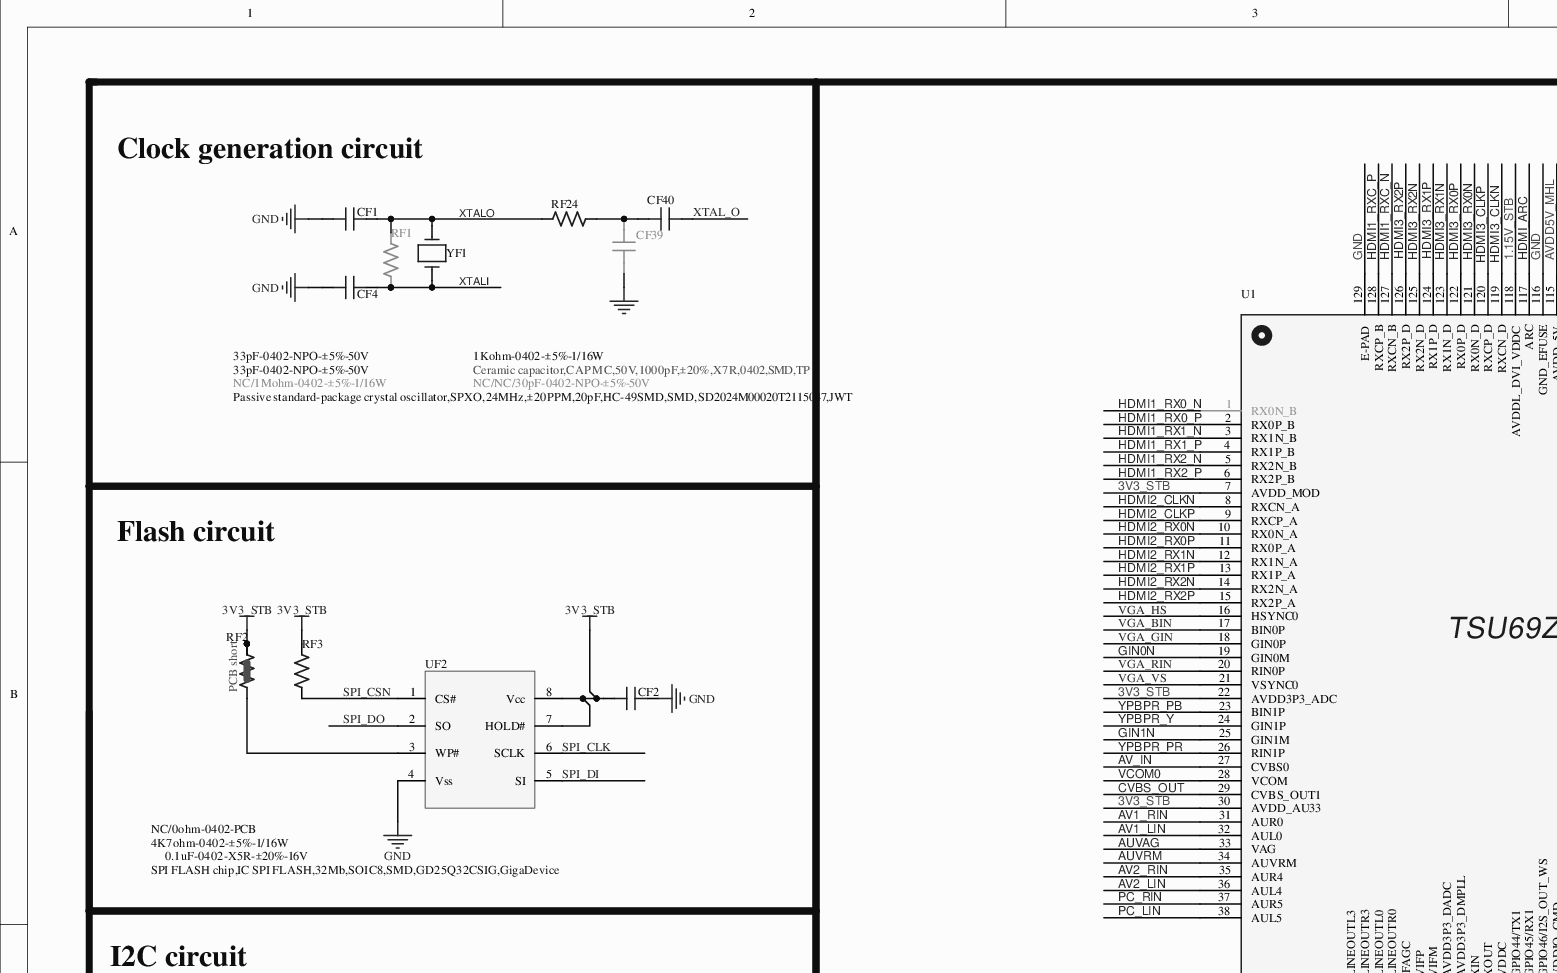
[diagram p0: MISC84438-8.SchDoc, top left]
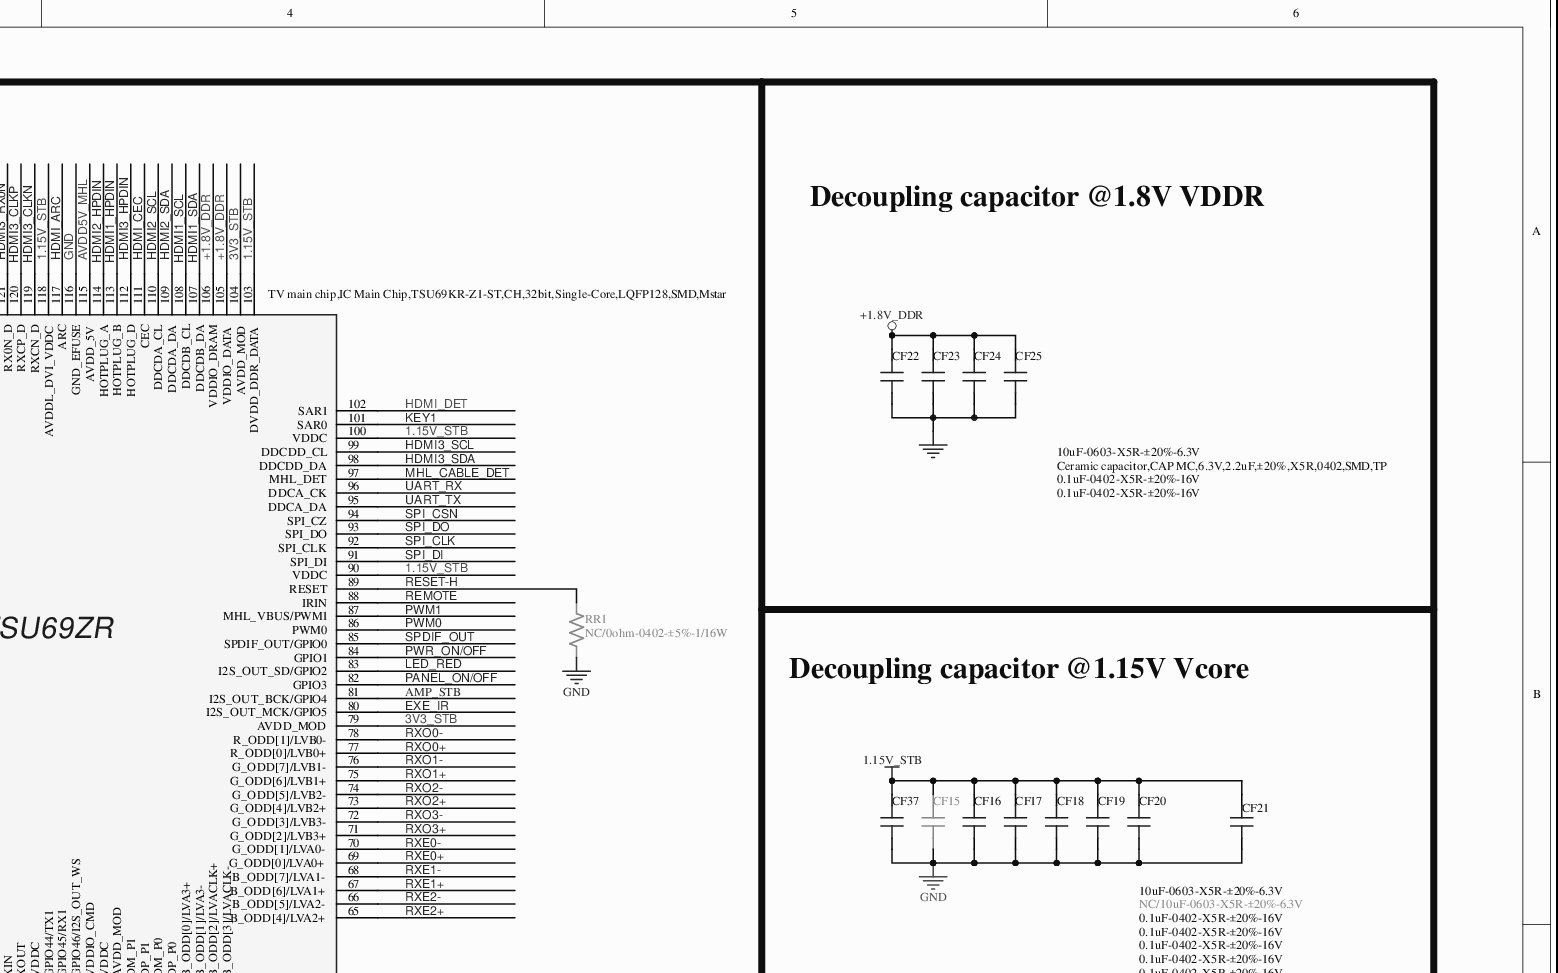
[diagram p1: MISC84438-8.SchDoc, top right]
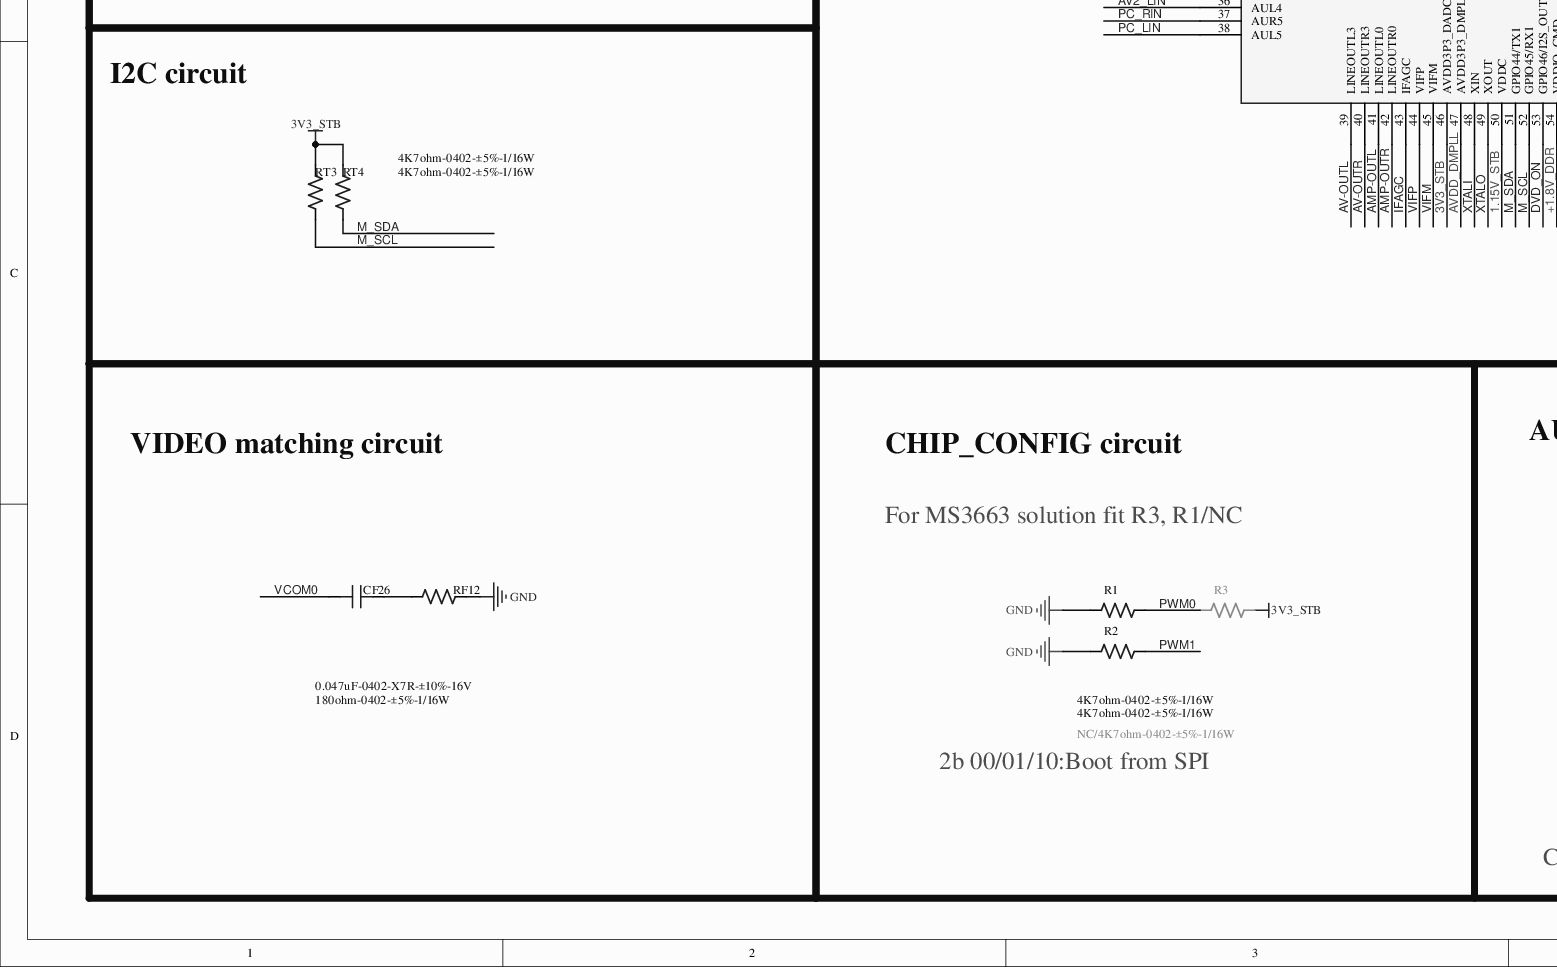
[diagram p2: MISC84438-8.SchDoc, bottom left]
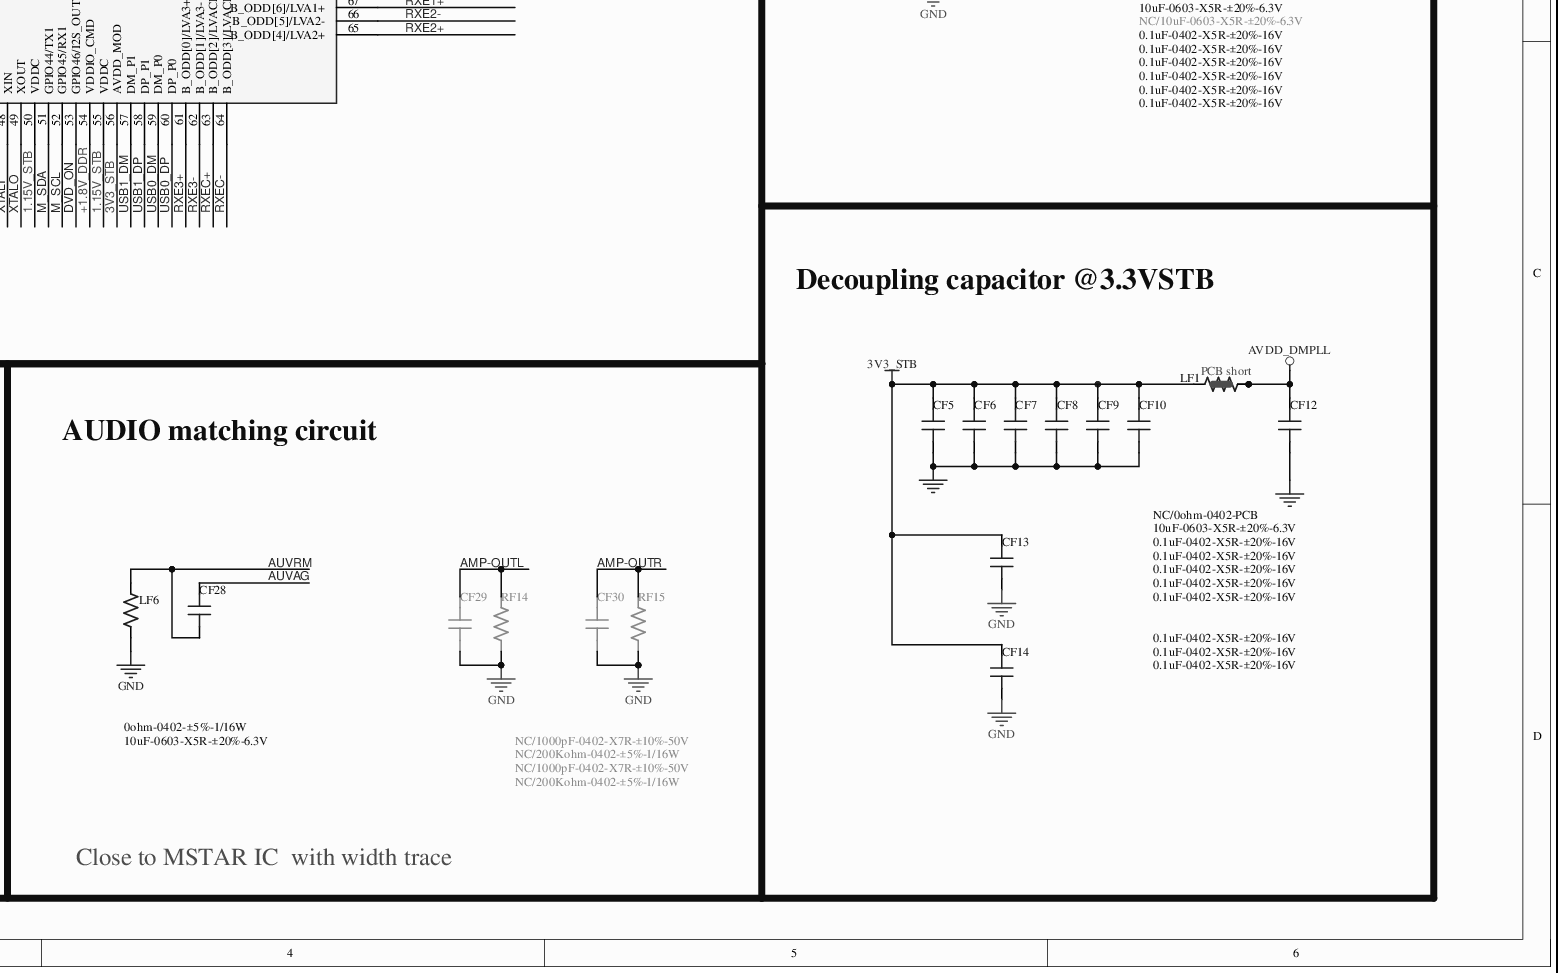
[diagram p3: MISC84438-8.SchDoc, bottom right]
# Altium project MISC84438-18.PrjPCB (part 4 of 8)

## Sheet MISC84438-8.SchDoc
size 558 x 342 mm

### Parts
CF1  33pF-0402-NPO-±5%-50V  [C0402]
CF2  0.1uF-0402-X5R-±20%-16V  [C0402]
CF4  33pF-0402-NPO-±5%-50V  [C0402]
CF5  10uF-0603-X5R-±20%-6.3V  [C0603]
CF6  0.1uF-0402-X5R-±20%-16V  [C0402]
CF7  0.1uF-0402-X5R-±20%-16V  [C0402]
CF8  0.1uF-0402-X5R-±20%-16V  [C0402]
CF9  0.1uF-0402-X5R-±20%-16V  [C0402]
CF10  0.1uF-0402-X5R-±20%-16V  [C0402]
CF12  0.1uF-0402-X5R-±20%-16V  [C0402]
CF13  0.1uF-0402-X5R-±20%-16V  [C0402]
CF14  0.1uF-0402-X5R-±20%-16V  [C0402]
CF15  NC/10uF-0603-X5R-±20%-6.3V  [C0603]
CF16  0.1uF-0402-X5R-±20%-16V  [C0402]
CF17  0.1uF-0402-X5R-±20%-16V  [C0402]
CF18  0.1uF-0402-X5R-±20%-16V  [C0402]
CF19  0.1uF-0402-X5R-±20%-16V  [C0402]
CF20  0.1uF-0402-X5R-±20%-16V  [C0402]
CF21  0.1uF-0402-X5R-±20%-16V  [C0402]
CF22  10uF-0603-X5R-±20%-6.3V  [C0603]
CF23  Ceramic capacitor,CAP MC,6.3V,2.2uF,±20%,X5R,0402,SMD,TP  [C0402]
CF24  0.1uF-0402-X5R-±20%-16V  [C0402]
CF25  0.1uF-0402-X5R-±20%-16V  [C0402]
CF26  0.047uF-0402-X7R-±10%-16V  [C0402]
CF28  10uF-0603-X5R-±20%-6.3V  [C0603]
CF29  NC/1000pF-0402-X7R-±10%-50V  [C0402]
CF30  NC/1000pF-0402-X7R-±10%-50V  [C0402]
CF37  10uF-0603-X5R-±20%-6.3V  [C0603]
CF39  NC/NC/30pF-0402-NPO-±5%-50V  [C0402]
CF40  Ceramic capacitor,CAP MC,50V,1000pF,±20%,X7R,0402,SMD,TP  [C0402]
LF1  NC/0ohm-0402-PCB  [R0402SC]
LF6  0ohm-0402-±5%-1/16W  [R0402]
R1  4K7ohm-0402-±5%-1/16W  [R0402]
R2  4K7ohm-0402-±5%-1/16W  [R0402]
R3  NC/4K7ohm-0402-±5%-1/16W  [R0402]
RF1  NC/1Mohm-0402-±5%-1/16W  [R0402]
RF2  NC/0ohm-0402-PCB  [R0402SC]
RF3  4K7ohm-0402-±5%-1/16W  [R0402]
RF12  180ohm-0402-±5%-1/16W  [R0402]
RF14  NC/200Kohm-0402-±5%-1/16W  [R0402]
RF15  NC/200Kohm-0402-±5%-1/16W  [R0402]
RF24  1Kohm-0402-±5%-1/16W  [R0402]
RR1  NC/0ohm-0402-±5%-1/16W  [R0402]
RT3  4K7ohm-0402-±5%-1/16W  [R0402]
RT4  4K7ohm-0402-±5%-1/16W  [R0402]
U1  TV main chip,IC Main Chip,TSU69KR-Z1-ST,CH,32bit,Single-Core,LQFP128,SMD,Mstar  [QFP128/0.4-5]
UF2  SPI FLASH chip,IC SPI FLASH,32Mb,SOIC8,SMD,GD25Q32CSIG,GigaDevice  [SOIC8]
YF1  Passive standard-package crystal oscillator,SPXO,24MHz,±20PPM,20pF,HC-49SMD,SMD,SD2024M00020T2115047,JWT  [XTAL-S-1]

### Blocks framed on the sheet
Flash circuit: CF2 RF2 RF3 UF2
VIDEO matching circuit: CF26 RF12

### Nets
1.15V_STB: CF15.1 CF16.2 CF17.2 CF18.2 CF19.2 CF20.2 CF21.2 CF37.1 U1.50(VDDC) U1.55(VDDC) U1.90(VDDC) U1.100(VDDC) U1.103(DVDD_DDR_DATA) U1.118(AVDDL_DVI_VDDC)
3V3_STB: CF2.2 CF5.1 CF6.2 CF7.2 CF8.2 CF9.2 CF10.2 CF13.2 CF14.2 LF1.1 R3.2 RF2.2 RF2.3 RF3.2 RT3.1 RT4.1 U1.7(AVDD_MOD) U1.22(AVDD3P3_ADC) U1.30(AVDD_AU33) U1.46(AVDD3P3_DADC) U1.56(AVDD_MOD) U1.79(AVDD_MOD) U1.104(AVDD_MOD) UF2.7(HOLD#) UF2.8(Vcc)
+1.8V_DDR: CF22.1 CF23.2 CF24.2 CF25.2 U1.54(VDDIO_CMD) U1.105(VDDIO_DATA) U1.106(VDDIO_DRAM)
AVDD_DMPLL: CF12.2 LF1.2 LF1.3 U1.47(AVDD3P3_DMPLL)
GND: CF1.1 CF2.1 CF4.1 CF5.2 CF6.1 CF7.1 CF8.1 CF9.1 CF10.1 CF12.1 CF13.1 CF14.1 CF15.2 CF16.1 CF17.1 CF18.1 CF19.1 CF20.1 CF21.1 CF22.2 CF23.1 CF24.1 CF25.1 CF29.2 CF30.2 CF37.2 CF39.1 LF6.1 R1.2 R2.2 RF12.2 RF14.1 RF15.1 RR1.1 U1.116(GND_EFUSE) U1.129(E-PAD) UF2.4(Vss)
AMP-OUTL: CF29.1 RF14.2 U1.41(LINEOUTL0)
AMP-OUTR: CF30.1 RF15.2 U1.42(LINEOUTR0)
AMP_STB: U1.81(I2S_OUT_BCK/GPIO4)
AUVAG: CF28.2 U1.33(VAG)
AUVRM: CF28.1 LF6.2 U1.34(AUVRM)
AV1_LIN: U1.32(AUL0)
AV1_RIN: U1.31(AUR0)
AV2_LIN: U1.36(AUL4)
AV2_RIN: U1.35(AUR4)
AV-OUTL: U1.39(LINEOUTL3)
AV-OUTR: U1.40(LINEOUTR3)
AV_IN: U1.27(CVBS0)
AVDD5V_MHL: U1.115(AVDD_5V)
CVBS_OUT: U1.29(CVBS_OUT1)
DVD_ON: U1.53(GPIO46/I2S_OUT_WS)
EXE_IR: U1.80(I2S_OUT_MCK/GPIO5)
GIN0N: U1.19(GIN0M)
GIN1N: U1.25(GIN1M)
HDMI1_HPDIN: U1.113(HOTPLUG_B)
HDMI1_RX0_N: U1.1(RX0N_B)
HDMI1_RX0_P: U1.2(RX0P_B)
HDMI1_RX1_N: U1.3(RX1N_B)
HDMI1_RX1_P: U1.4(RX1P_B)
HDMI1_RX2_N: U1.5(RX2N_B)
HDMI1_RX2_P: U1.6(RX2P_B)
HDMI1_RXC_N: U1.127(RXCN_B)
HDMI1_RXC_P: U1.128(RXCP_B)
HDMI1_SCL: U1.108(DDCDB_CL)
HDMI1_SDA: U1.107(DDCDB_DA)
HDMI2_CLKN: U1.8(RXCN_A)
HDMI2_CLKP: U1.9(RXCP_A)
HDMI2_HPDIN: U1.114(HOTPLUG_A)
HDMI2_RX0N: U1.10(RX0N_A)
HDMI2_RX0P: U1.11(RX0P_A)
HDMI2_RX1N: U1.12(RX1N_A)
HDMI2_RX1P: U1.13(RX1P_A)
HDMI2_RX2N: U1.14(RX2N_A)
HDMI2_RX2P: U1.15(RX2P_A)
HDMI2_SCL: U1.110(DDCDA_CL)
HDMI2_SDA: U1.109(DDCDA_DA)
HDMI3_CLKN: U1.119(RXCN_D)
HDMI3_CLKP: U1.120(RXCP_D)
HDMI3_HPDIN: U1.112(HOTPLUG_D)
HDMI3_RX0N: U1.121(RX0N_D)
HDMI3_RX0P: U1.122(RX0P_D)
HDMI3_RX1N: U1.123(RX1N_D)
HDMI3_RX1P: U1.124(RX1P_D)
HDMI3_RX2N: U1.125(RX2N_D)
HDMI3_RX2P: U1.126(RX2P_D)
HDMI3_SCL: U1.99(DDCDD_CL)
HDMI3_SDA: U1.98(DDCDD_DA)
HDMI_ARC: U1.117(ARC)
HDMI_CEC: U1.111(CEC)
HDMI_DET: U1.102(SAR1)
IFAGC: U1.43(IFAGC)
KEY1: U1.101(SAR0)
LED_RED: U1.83(I2S_OUT_SD/GPIO2)
M_SCL: RT3.2 U1.52(GPIO45/RX1)
M_SDA: RT4.2 U1.51(GPIO44/TX1)
MHL_CABLE_DET: U1.97(MHL_DET)
PANEL_ON/OFF: U1.82(GPIO3)
PC_LIN: U1.38(AUL5)
PC_RIN: U1.37(AUR5)
PWM0: R1.1 R3.1 U1.86(PWM0)
PWM1: R2.1 U1.87(MHL_VBUS/PWM1)
PWR_ON/OFF: U1.84(GPIO1)
REMOTE: U1.88(IRIN)
RESET-H: RR1.2 U1.89(RESET)
RXE0+: U1.69(G_ODD[0]/LVA0+)
RXE0-: U1.70(G_ODD[1]/LVA0-)
RXE1+: U1.67(B_ODD[6]/LVA1+)
RXE1-: U1.68(B_ODD[7]/LVA1-)
RXE2+: U1.65(B_ODD[4]/LVA2+)
RXE2-: U1.66(B_ODD[5]/LVA2-)
RXE3+: U1.61(B_ODD[0]/LVA3+)
RXE3-: U1.62(B_ODD[1]/LVA3-)
RXEC+: U1.63(B_ODD[2]/LVACLK+)
RXEC-: U1.64(B_ODD[3]/LVACLK-)
RXO0+: U1.77(R_ODD[0]/LVB0+)
RXO0-: U1.78(R_ODD[1]/LVB0-)
RXO1+: U1.75(G_ODD[6]/LVB1+)
RXO1-: U1.76(G_ODD[7]/LVB1-)
RXO2+: U1.73(G_ODD[4]/LVB2+)
RXO2-: U1.74(G_ODD[5]/LVB2-)
RXO3+: U1.71(G_ODD[2]/LVB3+)
RXO3-: U1.72(G_ODD[3]/LVB3-)
SPDIF_OUT: U1.85(SPDIF_OUT/GPIO0)
SPI_CLK: U1.92(SPI_CLK) UF2.6(SCLK)
SPI_CSN: RF3.1 U1.94(SPI_CZ) UF2.1(CS#)
SPI_DI: U1.91(SPI_DI) UF2.5(SI)
SPI_DO: U1.93(SPI_DO) UF2.2(SO)
UART_RX: U1.96(DDCA_CK)
UART_TX: U1.95(DDCA_DA)
USB0_DM: U1.59(DM_P0)
USB0_DP: U1.60(DP_P0)
USB1_DM: U1.57(DM_P1)
USB1_DP: U1.58(DP_P1)
VCOM0: CF26.1 U1.28(VCOM)
VGA_BIN: U1.17(BIN0P)
VGA_GIN: U1.18(GIN0P)
VGA_HS: U1.16(HSYNC0)
VGA_RIN: U1.20(RIN0P)
VGA_VS: U1.21(VSYNC0)
VIFM: U1.45(VIFM)
VIFP: U1.44(VIFP)
XTAL_O: CF40.1
XTALI: CF4.2 RF1.1 U1.48(XIN) YF1.1
XTALO: CF1.2 RF1.2 RF24.2 U1.49(XOUT) YF1.2
YPBPR_PB: U1.23(BIN1P)
YPBPR_PR: U1.26(RIN1P)
YPBPR_Y: U1.24(GIN1P)
NetCF26_2: CF26.2 RF12.1
NetCF39_2: CF39.2 CF40.2 RF24.1
NetRF2_1: RF2.1 UF2.3(WP#)

### Notes on the sheet
- Clock generation circuit
- Decoupling capacitor @1.8V VDDR
- Decoupling capacitor @1.15V Vcore
- I2C circuit
- Decoupling capacitor @3.3VSTB
- AUDIO matching circuit
- CHIP_CONFIG circuit
- For MS3663 solution fit R3, R1/NC
- 2b 00/01/10:Boot from SPI
- Close to MSTAR IC  with width trace

### Library data of the parts
CF1 CF4 = 33pF-0402-NPO-±5%-50V-D
CF2 CF7-CF10 CF12-CF14 CF17 = 0.1uF-0402-Y5V-+80%-20%-16V-D
CF5 CF15 CF22 CF28 CF37 = 10uF-0603-X5R-±20%-6.3V-D
CF6 CF16 CF18-CF21 CF23-CF25 = 1uF-0402-X5R-±20%-6.3V-D
CF26 = 0.047uF-0402-X7R-±10%-16V-D
CF29 CF30 = 1000pF-0402-X7R-±10%-50V-D
CF39 CF40 = 30pF-0402-NPO-±5%-50V-D
LF1 RF2 = 0ohm-0402-PCB-D
LF6 RR1 = 0ohm-0402-±5%-1/16W-D
R1-R3 RF3 RT3 RT4 = 4K7ohm-0402-±5%-1/16W-D
RF1 = 1Mohm-0402-±5%-1/16W-D
RF12 = 68ohm-0402-±5%-1/16W-D
RF14 RF15 = 200Kohm-0402-±5%-1/16W-D
RF24 = 1Kohm-0402-±5%-1/16W-D
U1 = TSU69ZR-D
UF2 = SPI FLASH 芯片,IC SPI FLASH,32Mb,SOIC8,SMD,GD25Q32CSIG,GigaDevice-D
YF1 = 24MHz-±20PPM-20PF-HC-49S-SMD-D

## Sheet MISC84438-9.SchDoc
size 431 x 292 mm
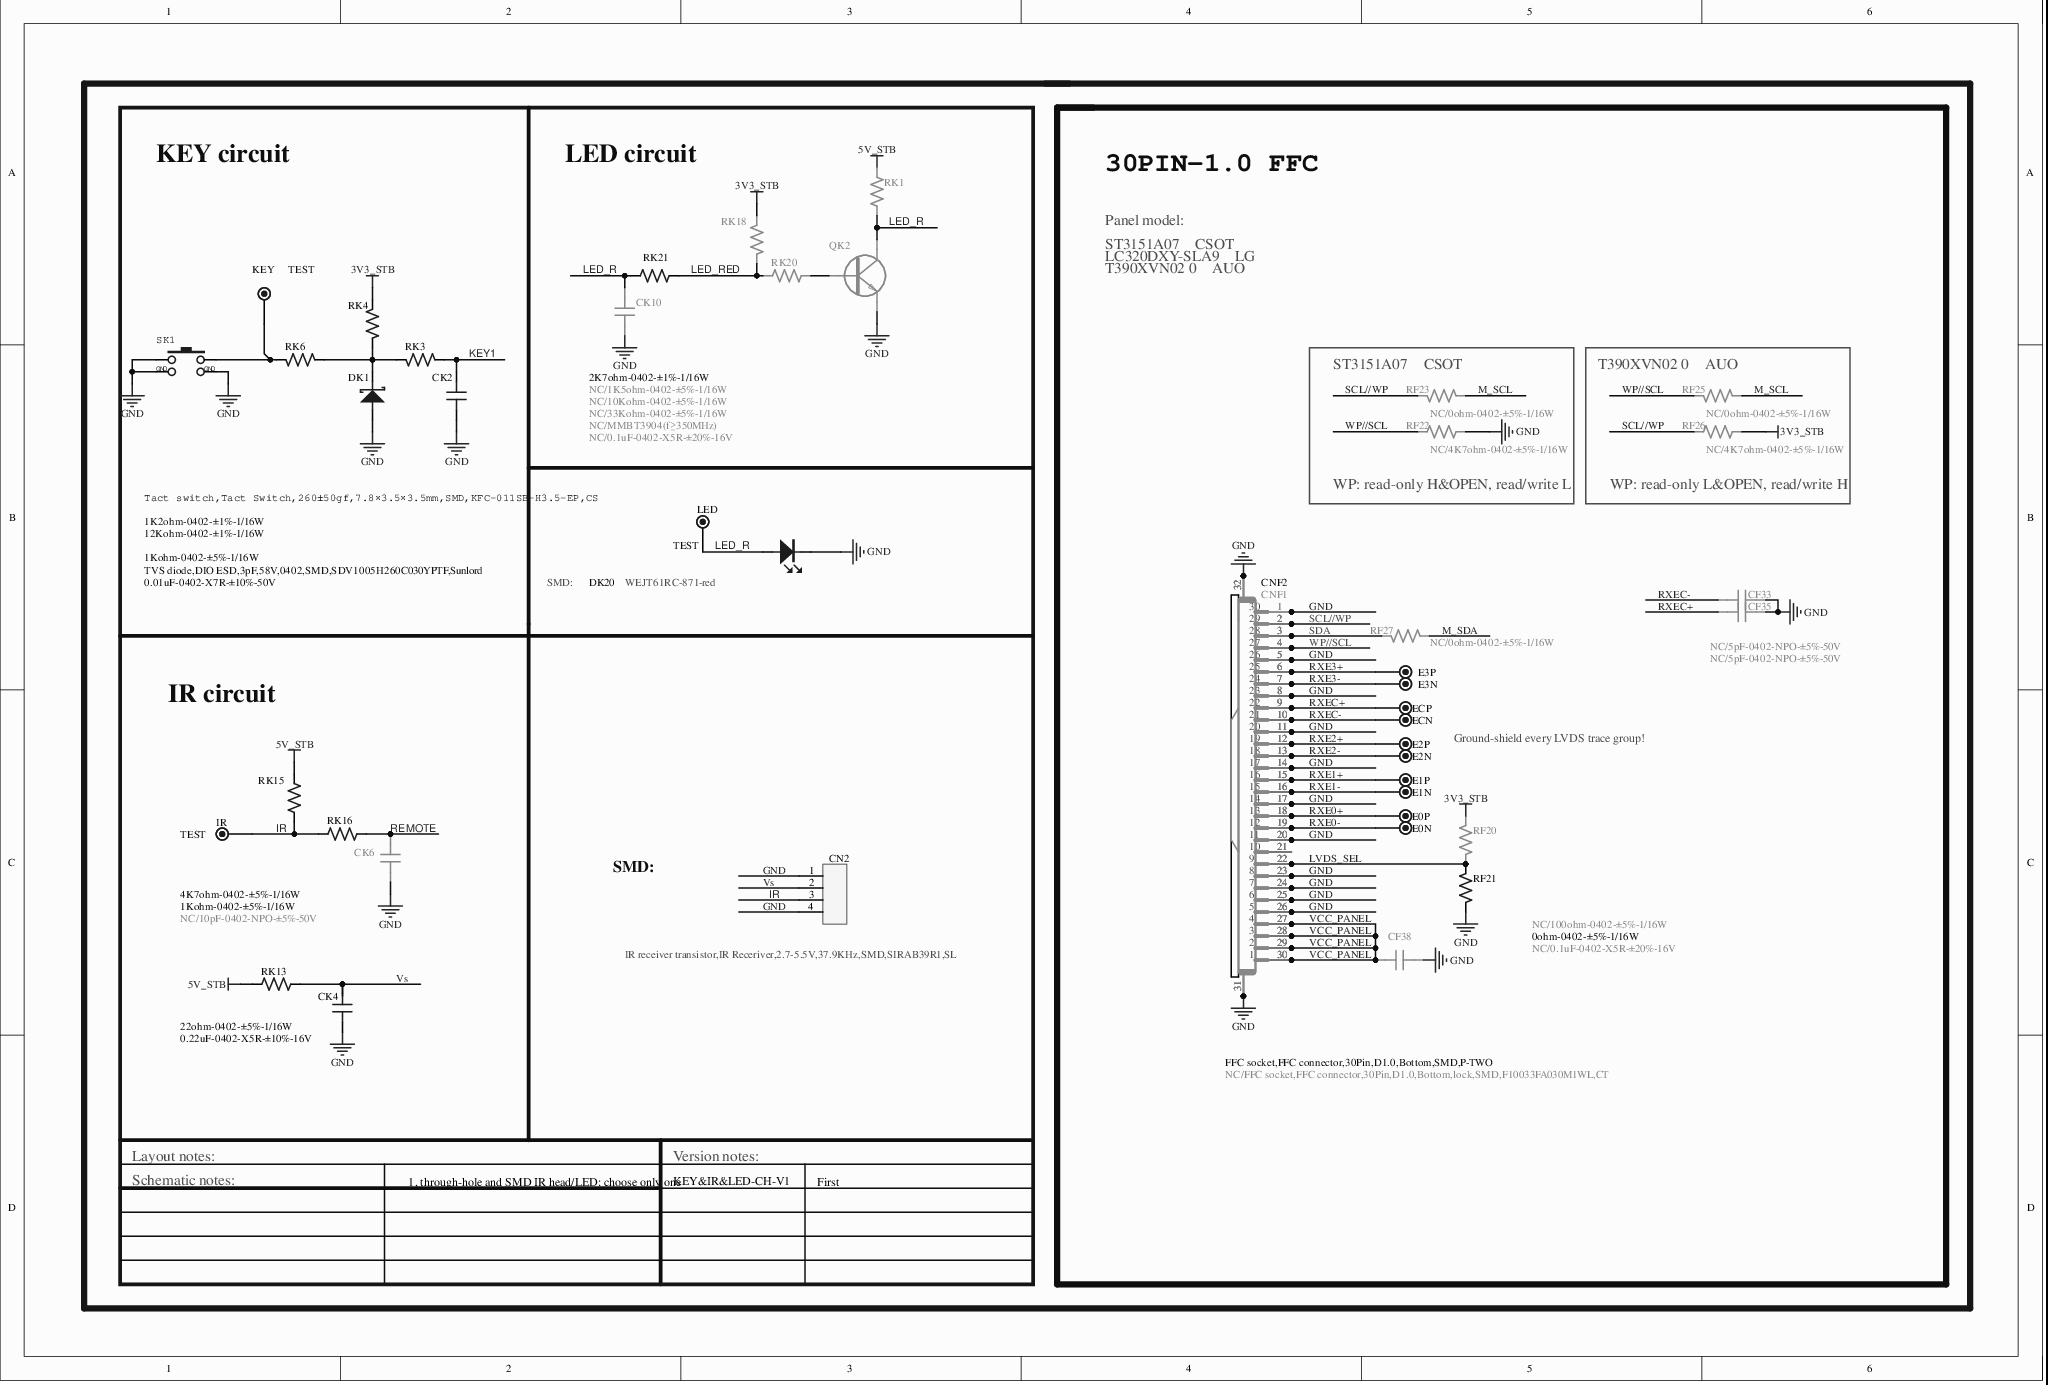
[diagram p4: MISC84438-9.SchDoc]

### Parts
CF33  NC/5pF-0402-NPO-±5%-50V  [C0402]
CF35  NC/5pF-0402-NPO-±5%-50V  [C0402]
CF38  NC/0.1uF-0402-X5R-±20%-16V  [C0402]
CK2  0.01uF-0402-X7R-±10%-50V  [C0402]
CK4  0.22uF-0402-X5R-±10%-16V  [C0402]
CK6  NC/10pF-0402-NPO-±5%-50V  [C0402]
CK10  NC/0.1uF-0402-X5R-±20%-16V  [C0402]
CN2  IR receiver transistor,IR Receriver,2.7-5.5V,37.9KHz,SMD,SIRAB39R1,SL  [REMOTE-HS-1]
CNF1  NC/FFC socket,FFC connector,30Pin,D1.0,Bottom,lock,SMD,F10033FA030M1WL,CT  [FFC30H/1.0S-7]
CNF2  FFC socket,FFC connector,30Pin,D1.0,Bottom,SMD,P-TWO  [FFC30H/1.0S-1]
DK1  TVS diode,DIO ESD,3pF,58V,0402,SMD,SDV1005H260C030YPTF,Sunlord  [DIODE-S0402]
DK20  WEJT61RC-871-red  [DIODE-S0603]
E0N  TEST  [TP]  (value not drawn)
E0P  TEST  [TP]  (value not drawn)
E1N  TEST  [TP]  (value not drawn)
E1P  TEST  [TP]  (value not drawn)
E2N  TEST  [TP]  (value not drawn)
E2P  TEST  [TP]  (value not drawn)
E3N  TEST  [TP]  (value not drawn)
E3P  TEST  [TP]  (value not drawn)
ECN  TEST  [TP]  (value not drawn)
ECP  TEST  [TP]  (value not drawn)
IR  TEST  [TP]
KEY  TEST  [TP]
LED  TEST  [TP]
QK2  NC/MMBT3904(f≥350MHz)  [SOT-23]
RF20  NC/100ohm-0402-±5%-1/16W  [R0402]
RF21  0ohm-0402-±5%-1/16W  [R0402]
RF22  NC/4K7ohm-0402-±5%-1/16W  [R0402]
RF23  NC/0ohm-0402-±5%-1/16W  [R0402]
RF25  NC/0ohm-0402-±5%-1/16W  [R0402]
RF26  NC/4K7ohm-0402-±5%-1/16W  [R0402]
RF27  NC/0ohm-0402-±5%-1/16W  [R0402]
RK1  NC/1K5ohm-0402-±5%-1/16W  [R0402]
RK3  1Kohm-0402-±5%-1/16W  [R0402]
RK4  12Kohm-0402-±1%-1/16W  [R0402]
RK6  1K2ohm-0402-±1%-1/16W  [R0402]
RK13  22ohm-0402-±5%-1/16W  [R0402]
RK15  4K7ohm-0402-±5%-1/16W  [R0402]
RK16  1Kohm-0402-±5%-1/16W  [R0402]
RK18  NC/33Kohm-0402-±5%-1/16W  [R0402]
RK20  NC/10Kohm-0402-±5%-1/16W  [R0402]
RK21  2K7ohm-0402-±1%-1/16W  [R0402]
SK1  Tact switch,Tact Switch,260±50gf,7.8×3.5×3.5mm,SMD,KFC-011SB-H3.5-EP,CS  [KEY-HS-5]

### Nets
3V3_STB: RF20.2 RF26.1 RK4.2 RK18.2
5V_STB: RK1.2 RK13.1 RK15.1
GND: CF33.1 CF35.1 CF38.2 CK2.2 CK4.2 CK6.1 CK10.1 CN2.1 CN2.4 CNF1.1 CNF1.5 CNF1.8 CNF1.11 CNF1.14 CNF1.17 CNF1.20 CNF1.23 CNF1.24 CNF1.25 CNF1.26 CNF1.31 CNF1.32 CNF2.1 CNF2.5 CNF2.8 CNF2.11 CNF2.14 CNF2.17 CNF2.20 CNF2.23 CNF2.24 CNF2.25 CNF2.26 CNF2.31 CNF2.32 DK1.A DK20.K QK2.E RF21.1 RF22.1 SK1.1 SK1.3 SK1.4(GND)
VCC_PANEL: CF38.1 CNF1.27 CNF1.28 CNF1.29 CNF1.30 CNF2.27 CNF2.28 CNF2.29 CNF2.30
IR: CN2.3 IR.1 RK15.2 RK16.2
KEY1: CK2.1 RK3.1
LED_R: CK10.2 DK20.A LED.1 QK2.C RK1.1 RK21.2
LED_RED: RK18.1 RK20.2 RK21.1
LVDS_SEL: CNF1.22 CNF2.22 RF20.1 RF21.2
M_SCL: RF23.1 RF25.1
M_SDA: RF27.1
REMOTE: CK6.2 RK16.1
RXE0+: CNF1.18 CNF2.18 E0P.1
RXE0-: CNF1.19 CNF2.19 E0N.1
RXE1+: CNF1.15 CNF2.15 E1P.1
RXE1-: CNF1.16 CNF2.16 E1N.1
RXE2+: CNF1.12 CNF2.12 E2P.1
RXE2-: CNF1.13 CNF2.13 E2N.1
RXE3+: CNF1.6 CNF2.6 E3P.1
RXE3-: CNF1.7 CNF2.7 E3N.1
RXEC+: CF35.2 CNF1.9 CNF2.9 ECP.1
RXEC-: CF33.2 CNF1.10 CNF2.10 ECN.1
SCL//WP: CNF1.2 CNF2.2 RF23.2 RF26.2
SDA: CNF1.3 CNF2.3 RF27.2
Vs: CK4.1 CN2.2 RK13.2
WP//SCL: CNF1.4 CNF2.4 RF22.2 RF25.2
NetCNF1_21: CNF1.21 CNF2.21
NetDK1_K: DK1.K RK3.2 RK4.1 RK6.1
NetKEY_1: KEY.1 RK6.2 SK1.2
NetQK2_B: QK2.B RK20.1

### Notes on the sheet
- KEY circuit
- LED circuit
- 30PIN-1.0 FFC
- Panel model:
- LC320DXY-SLA9    LG
- ST3151A07    CSOT
- T390XVN02 0    AUO
- (near RF23) ST3151A07    CSOT
- (near RF25) T390XVN02 0    AUO
- (near RF22) WP: read-only H&OPEN, read/write L
- (near RF26) WP: read-only L&OPEN, read/write H
- SMD:
- 29
- 30
- 24
- 25
- 26
- 27
- 28
- IR circuit
- 19
- 20
- 21
- 22
- 23
- Ground-shield every LVDS trace group!
- 14
- 15
- 16
- 17
- 18
- 9
- 10
- 11
- 12
- 13
- 4
- 5
- 6
- 7
- 8
- 1
- 2
- 3
- Layout notes:
- Version notes:
- Schematic notes:
- 1, through-hole and SMD IR head/LED: choose only one
- KEY&IR&LED-CH-V1
- First

### Library data of the parts
CF33 CF35 = 5pF-0402-NPO-±5%-50V-D
CF38 = 0.1uF-0402-X5R-±20%-16V-
CK2 = 0.01uF-0402-X7R-±10%-50V-D
CK4 CK10 = 0.1uF-0402-Y5V-+80%-20%-16V-D
CK6 = 10pF-0402-NPO-±5%-50V-D
CN2 = 红外接收三极管,Phototransistor,NPN,6.8×3×3.2mm,SMD,HS75438D,VISHAY-D
CNF1 = XXX.XXX.0004205-D: FFC socket,FFC connector,30Pin,D1.0,Bottom,lock,SMD,F10033FA030M1WL,CT-D
CNF2 = 196161-30041-3: CN-FFC socket-flip cover
DK1 = AVLC18S02003-D
DK20 = WEJT61RC-871-红色-D
QK2 = MMBT3904(f≥350MHz)-D-NPN: Q-NPN-#-#-#
RF20 = 100ohm-0402-±5%-1/16W-
RF21 RF23 RF25 RF27 = 1Kohm-0402-±5%-1/16W-
RF22 RF26 RK15 RK18 = 4K7ohm-0402-±5%-1/16W-D
RK1 = 22ohm-0402-±5%-1/16W-D
RK3 RK16 RK21 = 1Kohm-0402-±5%-1/16W-D
RK4 RK6 = 4K7ohm-0402-±1%-1/16W-D
RK13 = 100ohm-0402-±5%-1/16W-D
RK20 = 10Kohm-0402-±5%-1/16W-D
SK1 = TS06PW0-G35F(YF)-D